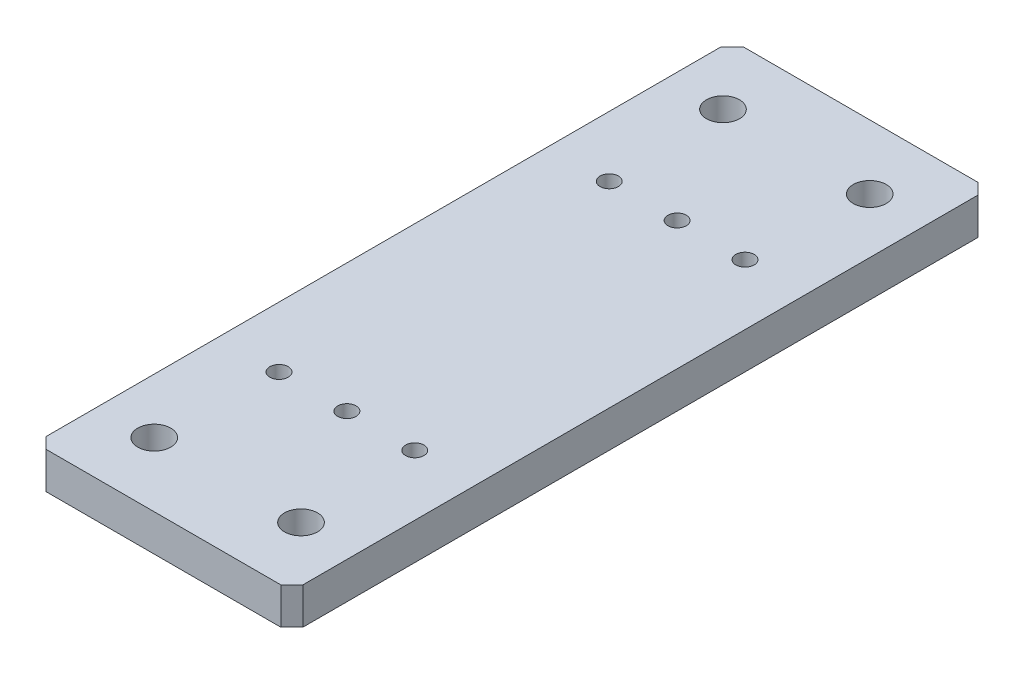
SolidWorks part; units mm, degrees
material "45#"
ref_plane "前基準面" through (0, 0, 0) normal (0, 0, 1) x (1, 0, 0)
ref_plane "上基準面" through (0, 0, 0) normal (0, 1, 0) x (1, 0, 0)
ref_plane "右基準面" through (0, 0, 0) normal (1, 0, 0) x (0, 0, -1)
sketch "草图1" plane through (0, 0, 0) normal (0, 1, 0) x (1, 0, 0)
  line L1 (-35, 95) -> (35, 95)
  line L2 (-35, 95) -> (-35, -95)
  line L3 (-35, -95) -> (35, -95)
  line L4 (35, 95) -> (35, -95)
  line L5 (-35, 95) -> (35, -95) construction
  line L6 (-35, -95) -> (35, 95) construction
  point P0 (0, 0)
  dimension "D1" = 190
  dimension "D2" = 70
extrude "凸台-拉伸1" add sketch "草图1" along normal blind 10
hole_wizard "M6 螺纹孔1" positions "草图2" profile "草图3" tap size "M6" standard "GB" end condition through all
sketch "草图2" plane through (0, 10, 0) normal (0, 1, 0) x (1, 0, 0)
  line L0 (0, 0) -> (-45.6674, 0) construction
  line L2 (0, 0) -> (0, 112.6662) construction
  point P0 (18.5, 45)
  point P2 (-18.5, 45)
  point P13 (0, 45)
  point P15 (0, -45)
  point P16 (-18.5, -45)
  point P17 (18.5, -45)
  dimension "D1" = 37
  dimension "D2" = 90
sketch "草图3" plane through (18.5, 10, -45) normal (1, 0, 0) x (0, 0, 1)
  line L0 (0, 0) -> (0, 10)
  line L1 (0, 10) -> (2.5, 10)
  line L2 (2.5, 10) -> (2.5, 0)
  line L5 (2.5, 0) -> (0, 0)
  line L11 (0, -6.35) -> (0, 107.95) construction
  dimension "通孔螺纹孔钻头直径" = 5
  dimension "通孔螺纹孔钻头深度" = 10
cosmetic thread "孔螺蚊线1" parameters "D2"=6
cosmetic thread "孔螺蚊线2" parameters "D2"=6
cosmetic thread "孔螺蚊线3" parameters "D2"=6
cosmetic thread "孔螺蚊线4" parameters "D2"=6
cosmetic thread "孔螺蚊线5" parameters "D2"=6
cosmetic thread "孔螺蚊线6" parameters "D2"=6
hole_wizard "Ø9.0 (9) 直径孔1" positions "草图4" profile "草图5" hole size "Ø9.0" standard "GB" end condition through all
sketch "草图4" plane through (0, 10, 0) normal (0, 1, 0) x (1, 0, 0)
  line L1 (0, 0) -> (0, 104.8704) construction
  line L3 (0, 0) -> (-39.9386, 0) construction
  point P0 (-20, 77.5)
  point P5 (20, 77.5)
  point P18 (20, -77.5)
  point P19 (-20, -77.5)
  dimension "D3" = 40
sketch "草图5" plane through (-20, 10, -77.5) normal (1, 0, 0) x (0, 0, 1)
  line L0 (0, 0) -> (0, 10)
  line L1 (0, 10) -> (4.5, 10)
  line L2 (4.5, 10) -> (4.5, 0)
  line L5 (4.5, 0) -> (0, 0)
  line L11 (0, -6.35) -> (0, 107.95) construction
  dimension "通孔孔直径" = 9
  dimension "通孔孔深度" = 10
chamfer "倒角1" distance 3 angle 45 4 edges at (-35, 5, -95) (35, 5, -95) (-35, 5, 95) (35, 5, 95)
